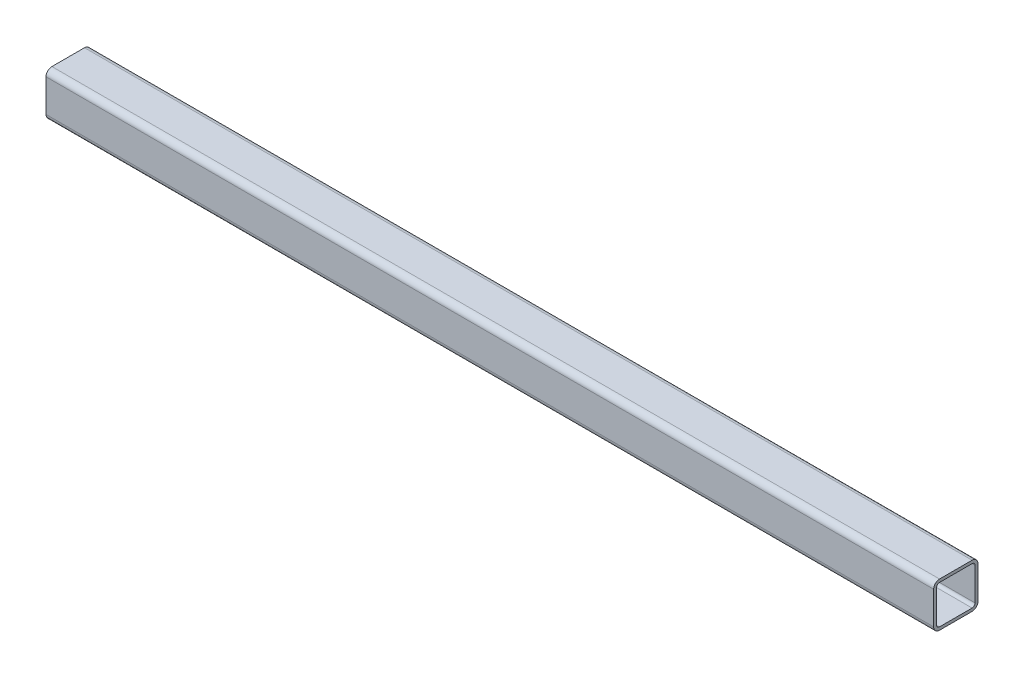
from build123d import *

# Parameters (mm, degrees)
GB_6728_1986_60_X_60_X_4_1_DEPTH = 1200


with BuildPart() as part:
    # Sketch11 → Gb／6728-1986方形空心型钢 60 X 60 X 4(1) (new body)
    with BuildSketch(Plane(origin=(-600, 0, 0), x_dir=(0, 0, -1), z_dir=(1, 0, 0))):
        with BuildLine():
            Line((-22, -30), (22, -30))
            ThreePointArc((22, -30), (27.656854249, -27.656854249), (30, -22))
            Line((30, -22), (30, 22))
            ThreePointArc((30, 22), (27.656854249, 27.656854249), (22, 30))
            Line((22, 30), (-22, 30))
            ThreePointArc((-22, 30), (-27.656854249, 27.656854249), (-30, 22))
            Line((-30, 22), (-30, -22))
            ThreePointArc((-30, -22), (-27.656854249, -27.656854249), (-22, -30))
        make_face()
        with BuildLine():
            Line((-22, -26), (22, -26))
            ThreePointArc((22, -26), (24.828427125, -24.828427125), (26, -22))
            Line((26, -22), (26, 22))
            ThreePointArc((26, 22), (24.828427125, 24.828427125), (22, 26))
            Line((22, 26), (-22, 26))
            ThreePointArc((-22, 26), (-24.828427125, 24.828427125), (-26, 22))
            Line((-26, 22), (-26, -22))
            ThreePointArc((-26, -22), (-24.828427125, -24.828427125), (-22, -26))
        make_face(mode=Mode.SUBTRACT)
    extrude(amount=GB_6728_1986_60_X_60_X_4_1_DEPTH)


solid = part.part
